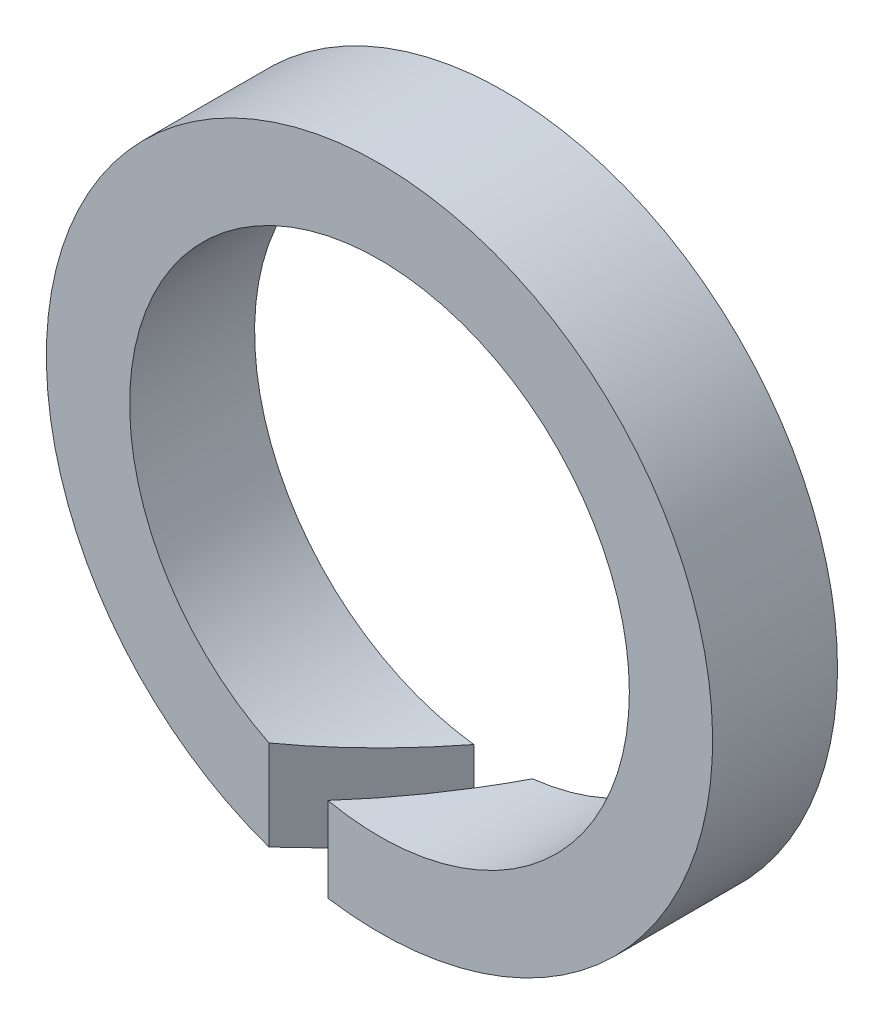
from build123d import *

# Parameters (mm, degrees)
SKETCH1_W          = 2
SKETCH1_H          = 3
CUT_EXTRUDE1_DEPTH = 23


with BuildPart() as part:
    # Sketch1 → Revolve1 (revolve)
    with BuildSketch(Plane(origin=(0, 0, 0), x_dir=(1, 0, 0), z_dir=(0, 1, 0))):
        with Locations((7, 5.564714504)):
            Rectangle(SKETCH1_W, SKETCH1_H)
    revolve(axis=Axis((0, 0, 0), (0, 0, -1)))

    # Sketch2 → Cut-Extrude1 (cut)
    with BuildSketch(Plane(origin=(0, 0, 0), x_dir=(1, 0, 0), z_dir=(0, 1, 0))):
        Polygon((-3.27585187, 3.09237347), (2.379628245, 11.930992665), (3.38205654, 11.289578756), (-2.273423575, 2.450959561), align=None)
    extrude(amount=-CUT_EXTRUDE1_DEPTH, mode=Mode.SUBTRACT)


solid = part.part
